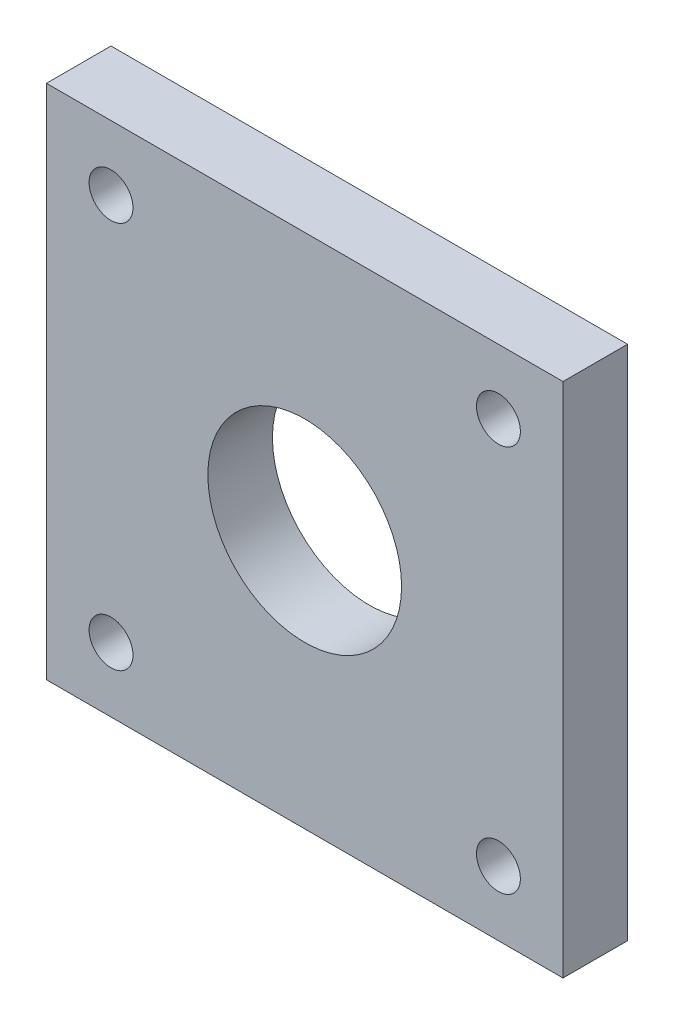
SolidWorks part; units mm, degrees
material "1023 碳钢板 (SS)"
ref_plane "Front Plane" through (0, 0, 0) normal (0, 0, 1) x (1, 0, 0)
ref_plane "Top Plane" through (0, 0, 0) normal (0, 1, 0) x (1, 0, 0)
ref_plane "Right Plane" through (0, 0, 0) normal (1, 0, 0) x (0, 0, -1)
sketch "Sketch1" plane through (0, 0, 0) normal (0, 0, 1) x (1, 0, 0)
  line L1 (40, 40) -> (-40, 40)
  line L2 (40, 40) -> (40, -40)
  line L3 (40, -40) -> (-40, -40)
  line L4 (-40, 40) -> (-40, -40)
  line L5 (40, 40) -> (-40, -40) construction
  line L6 (40, -40) -> (-40, 40) construction
  point P0 (0, 0)
  dimension "D1" = 80
  dimension "D2" = 80
extrude "Boss-Extrude1" add sketch "Sketch1" along normal blind 10
sketch "Sketch2" plane through (0, 0, 10) normal (0, 0, 1) x (1, 0, 0)
  line L1 (30, -30) -> (-30, -30) construction
  line L2 (30, -30) -> (30, 30) construction
  line L3 (30, 30) -> (-30, 30) construction
  line L4 (-30, -30) -> (-30, 30) construction
  line L5 (30, -30) -> (-30, 30) construction
  line L6 (30, 30) -> (-30, -30) construction
  point P0 (0, 0)
  dimension "D1" = 60
  dimension "D2" = 60
hole_wizard "M8 Tapped Hole1" positions "Sketch3" profile "Sketch4" tap size "M8" standard "ISO"
sketch "Sketch3" plane through (0, 0, 10) normal (0, 0, 1) x (1, 0, 0)
  point P0 (-30, 30)
  point P3 (30, 30)
  point P6 (30, -30)
  point P9 (-30, -30)
sketch "Sketch4" plane through (-30, 30, 10) normal (1, 0, 0) x (0, -1, 0)
  line L0 (0, 0) -> (0, 21.7929)
  line L1 (0, 21.7929) -> (3.4, 19.75)
  line L2 (3.4, 19.75) -> (3.4, 0)
  line L5 (3.4, 0) -> (0, 0)
  line L10 (0, 21.7929) -> (-3.4, 19.75) construction
  line L11 (0, -6.35) -> (0, 107.95) construction
  dimension "螺纹孔钻头直径" = 6.8
  dimension "螺纹孔钻头深度" = 19.75
  dimension "导头角度" = 118
cosmetic thread "Hole thread line 1"
cosmetic thread "Hole thread line 2"
cosmetic thread "Hole thread line 3"
cosmetic thread "Hole thread line 4"
sketch "Sketch5" plane through (0, 0, 10) normal (0, 0, 1) x (1, 0, 0)
  circle A0 centre (0, 0) radius 15
  dimension "D1" = 30
extrude "Cut-Extrude1" cut sketch "Sketch5" against normal blind 10
